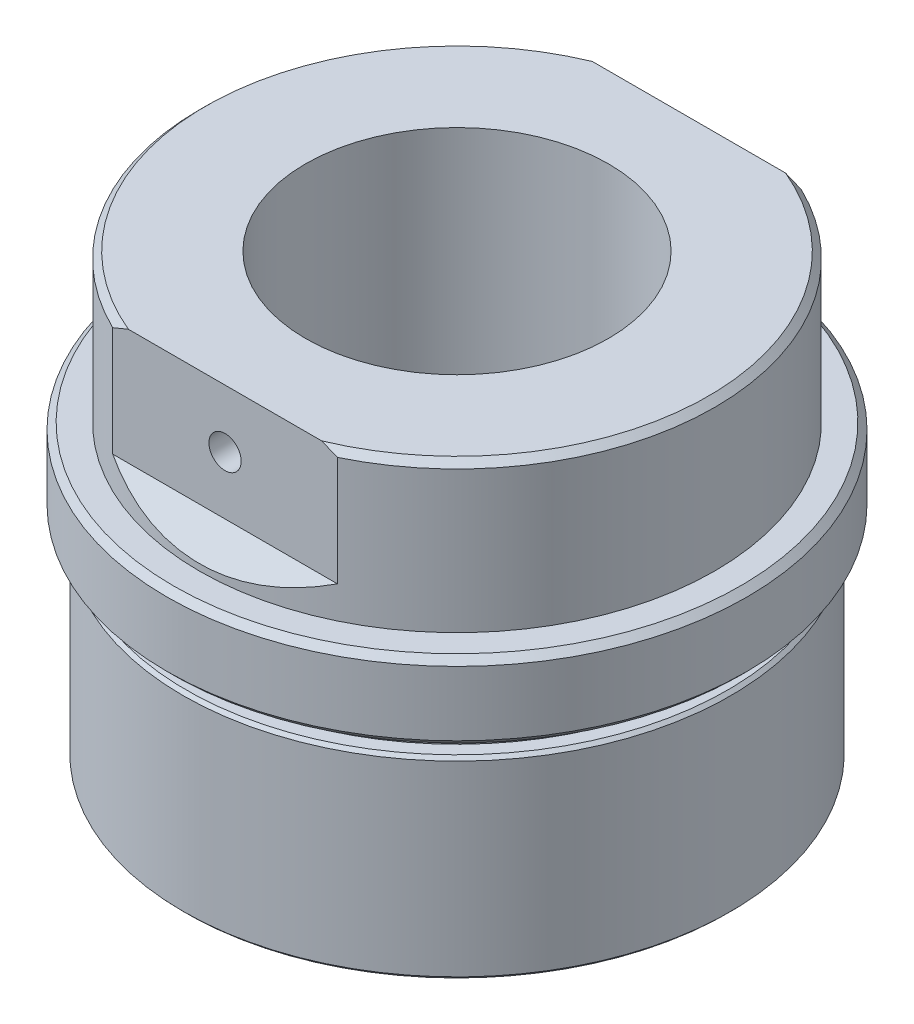
from build123d import *

# Parameters (mm, degrees)
SKETCH1_R               = 40
BOSS_EXTRUDE1_DEPTH     = 30
SKETCH2_R               = 18
BOSS_EXTRUDE2_DEPTH     = 60
SKETCH3_W               = 77.976815456
SKETCH3_H               = 25.992271819
SKETCH3_W_2             = 92.098600933
SKETCH3_H_2             = 25.173617588
CUT_EXTRUDE1_DEPTH      = 18
SKETCH7_R               = 42.5
BOSS_EXTRUDE3_DEPTH     = 38
SKETCH14_R              = 3
CUT_EXTRUDE3_DEPTH      = 63
CUT_EXTRUDE4_START      = -30
SKETCH15_R              = 67.080871601
SKETCH15_R_2            = 40
CUT_EXTRUDE4_DEPTH      = 3
SKETCH17_R              = 45
SKETCH17_R_2            = 16.642095107
BOSS_EXTRUDE4_DEPTH     = 10
CHAMFER1_SIZE           = 1
CUT_EXTRUDE5_DEPTH      = 111.227038425
CUT_EXTRUDE5_DEPTH_BACK = 111.227038425
SKETCH20_R              = 45
BOSS_EXTRUDE5_DEPTH     = 2
CHAMFER2_SIZE           = 1
CHAMFER3_SIZE           = 1
SKETCH21_R              = 3
CUT_EXTRUDE7_DEPTH      = 2
SKETCH22_R              = 18
CUT_EXTRUDE8_DEPTH      = 94.134311615
M52X5_0_TAPPED_HOLE1_D  = 47
BOSS_EXTRUDE6_START     = -33
SKETCH25_R              = 42.5
SKETCH25_R_2            = 34.471384151
BOSS_EXTRUDE6_DEPTH     = 33
SKETCH26_OUTSIDE_W      = 120.862
SKETCH26_OUTSIDE_H      = 120.862
SKETCH26_OUTSIDE_R      = 40
CUT_EXTRUDE9_DEPTH      = 3
CHAMFER4_SIZE           = 0.5
M6_TAPPED_HOLE1_D       = 5
M6_TAPPED_HOLE1_DEPTH   = 17
M6_TAPPED_HOLE1_TIP     = 1.502151548


with BuildPart() as part:
    # Sketch1 → Boss-Extrude1 (new body)
    with BuildSketch(Plane(origin=(0, 0, 0), x_dir=(1, 0, 0), z_dir=(0, 1, 0))):
        with Locations(Location((0, 0, 0), (0, 0, 270))):
            Circle(SKETCH1_R)
    extrude(amount=BOSS_EXTRUDE1_DEPTH)

    # Sketch2 → Boss-Extrude2 (add)
    with BuildSketch(Plane(origin=(0, 30, 0), x_dir=(1, 0, 0), z_dir=(0, 1, 0))):
        with Locations(Location((0, 0, 0), (0, 0, 270))):
            Circle(SKETCH2_R)
    extrude(amount=BOSS_EXTRUDE2_DEPTH)

    # Sketch3 → Cut-Extrude1 (cut)
    with BuildSketch(Plane(origin=(0, 30, 0), x_dir=(1, 0, 0), z_dir=(0, 1, 0))):
        with Locations((-2.353630913, 48.996135909)):
            Rectangle(SKETCH3_W, SKETCH3_H)
        with Locations((4.707261826, -48.586808794)):
            Rectangle(SKETCH3_W_2, SKETCH3_H_2)
    extrude(amount=-CUT_EXTRUDE1_DEPTH, mode=Mode.SUBTRACT)

    # Sketch7 → Boss-Extrude3 (add)
    with BuildSketch(Plane.XZ):
        with Locations(Location((0, 0, 0), (0, 0, 270))):
            Circle(SKETCH7_R)
    extrude(amount=BOSS_EXTRUDE3_DEPTH)

    # Sketch14 → Cut-Extrude3 (cut)
    with BuildSketch(Plane.XZ.offset(38)):
        with Locations(Location((0, 0, 0), (0, 0, 270))):
            Circle(SKETCH14_R)
    extrude(amount=-CUT_EXTRUDE3_DEPTH, mode=Mode.SUBTRACT)

    # Sketch15 → Cut-Extrude4 (cut)
    with BuildSketch(Plane.XZ.offset(38).offset(CUT_EXTRUDE4_START)):
        Circle(SKETCH15_R)
        with Locations(Location((0, 0, 0), (0, 0, 270))):
            Circle(SKETCH15_R_2, mode=Mode.SUBTRACT)
    extrude(amount=-CUT_EXTRUDE4_DEPTH, mode=Mode.SUBTRACT)

    # Sketch17 → Boss-Extrude4 (add)
    with BuildSketch(Plane.XZ.offset(5)):
        with Locations(Location((0, 0, 0), (0, 0, 270))):
            Circle(SKETCH17_R)
        Circle(SKETCH17_R_2, mode=Mode.SUBTRACT)
    extrude(amount=-BOSS_EXTRUDE4_DEPTH)

    # Chamfer1
    chamfer1_edges = [part.edges().sort_by_distance(p)[0] for p in [
        (40, 30, 0),
        (0, -38, 42.5),
        (0, -5, 45),
        (0, 90, -18),
        (-40, 30, 0),
    ]]
    chamfer(chamfer1_edges, length=CHAMFER1_SIZE)

    # Sketch18 → Cut-Extrude5 (cut, two sides: drawn at the far end of the back side and taken through both)
    with BuildSketch(Plane(origin=(0, 0, 0), x_dir=(0, 0, -1), z_dir=(1, 0, 0)).offset(-CUT_EXTRUDE5_DEPTH_BACK)):
        Polygon((-40, 12), (-40, 8), (-36, 12), align=None)
        Polygon((36, 12), (41.96059215, 12), (41.96059215, 6.03940785), align=None)
    extrude(amount=CUT_EXTRUDE5_DEPTH + CUT_EXTRUDE5_DEPTH_BACK, mode=Mode.SUBTRACT)

    # Sketch20 → Boss-Extrude5 (add)
    with BuildSketch(Plane(origin=(0, 5, 0), x_dir=(1, 0, 0), z_dir=(0, 1, 0))):
        with Locations(Location((0, 0, 0), (0, 0, 90))):
            Circle(SKETCH20_R)
    extrude(amount=BOSS_EXTRUDE5_DEPTH)

    # Chamfer2
    chamfer2_edges = [part.edges().sort_by_distance(p)[0] for p in [
        (0, 7, 45),
    ]]
    chamfer(chamfer2_edges, length=CHAMFER2_SIZE)

    # Chamfer3
    chamfer3_edges = [part.edges().sort_by_distance(p)[0] for p in [
        (0, -8, 42.5),
    ]]
    chamfer(chamfer3_edges, length=CHAMFER3_SIZE)

    # Sketch21 → Cut-Extrude7 (cut)
    with BuildSketch(Plane.XZ.offset(-5)):
        with Locations(Location((0, 0, 0), (0, 0, 270))):
            Circle(SKETCH21_R)
    extrude(amount=-CUT_EXTRUDE7_DEPTH, mode=Mode.SUBTRACT)

    # Sketch22 → Cut-Extrude8 (cut, through all)
    with BuildSketch(Plane(origin=(0, 30, 0), x_dir=(1, 0, 0), z_dir=(0, 1, 0))):
        Circle(SKETCH22_R)
    extrude(amount=CUT_EXTRUDE8_DEPTH, mode=Mode.SUBTRACT)

    # M52x5.0 Tapped Hole1 (through all)
    with Locations(Plane(origin=(0, 30, 0), x_dir=(1, 0, 0), z_dir=(0, 1, 0))):
        with Locations((0, 0)):
            Hole(M52X5_0_TAPPED_HOLE1_D / 2)

    # Sketch25 → Boss-Extrude6 (add)
    with BuildSketch(Plane.XZ.offset(38).offset(BOSS_EXTRUDE6_START)):
        with Locations(Location((0, 0, 0), (0, 0, 270))):
            Circle(SKETCH25_R)
        Circle(SKETCH25_R_2, mode=Mode.SUBTRACT)
    extrude(amount=BOSS_EXTRUDE6_DEPTH)

    # Sketch26 outside → Cut-Extrude9 (cut)
    with BuildSketch(Plane.XZ.offset(5)):
        Rectangle(SKETCH26_OUTSIDE_W, SKETCH26_OUTSIDE_H)
        with Locations(Location((0, 0, 0), (0, 0, 244.158067237))):
            Circle(SKETCH26_OUTSIDE_R, mode=Mode.SUBTRACT)
    extrude(amount=CUT_EXTRUDE9_DEPTH, mode=Mode.SUBTRACT)

    # Chamfer4
    chamfer4_edges = [part.edges().sort_by_distance(p)[0] for p in [
        (0, -38, 42.5),
        (0, -8, 42.5),
    ]]
    chamfer(chamfer4_edges, length=CHAMFER4_SIZE)

    # M6 Tapped Hole1
    with Locations(Plane.XY.offset(36)):
        with Locations((0, 21)):
            Hole(M6_TAPPED_HOLE1_D / 2, depth=M6_TAPPED_HOLE1_DEPTH)
            with Locations((0, 0, -(M6_TAPPED_HOLE1_DEPTH + M6_TAPPED_HOLE1_TIP / 2))):  # 118° drill point
                Cone(0, M6_TAPPED_HOLE1_D / 2, M6_TAPPED_HOLE1_TIP, mode=Mode.SUBTRACT)


solid = part.part
